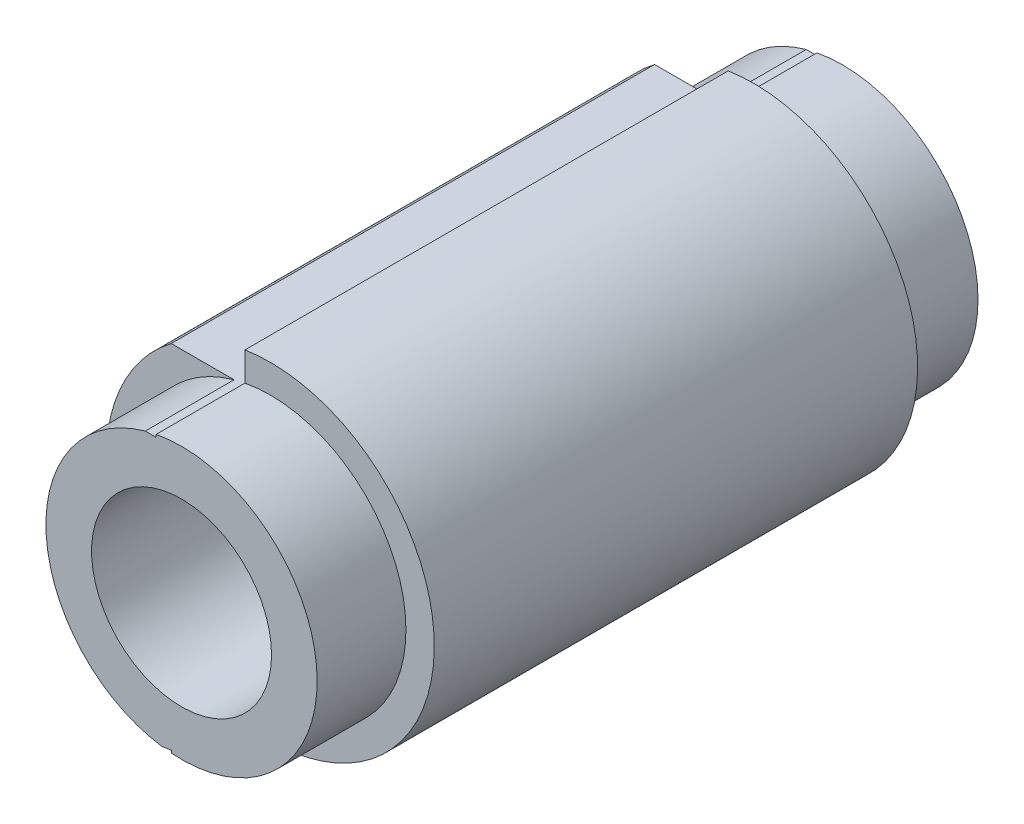
SolidWorks part; units mm, degrees
ref_plane "Front Plane" through (0, 0, 0) normal (0, 0, 1) x (1, 0, 0)
ref_plane "Top Plane" through (0, 0, 0) normal (0, 1, 0) x (1, 0, 0)
ref_plane "Right Plane" through (0, 0, 0) normal (1, 0, 0) x (0, 0, -1)
sketch "Sketch1" plane through (0, 0, 0) normal (0, 0, 1) x (1, 0, 0)
  line L0 (-40.1653, 53) -> (-10.3, 53)
  line L1 (-10.3, 53) -> (-10.3, 65.6975)
  line L2 (0, 0) -> (0, -98.1486) construction
  line L3 (-4.1281, -53.8236) -> (-2.1257, -66.466)
  line L4 (-4.1281, -53.8236) -> (-32.0797, -58.2507)
  circle A0 centre (0, 0) radius 36.5
  arc A1 (-40.1653, 53) -> (-32.0797, -58.2507) centre (0, 0) ccw
  arc A2 (-2.1257, -66.466) -> (-10.3, 65.6975) centre (0, 0) ccw
  dimension "D1" = 73
  dimension "D2" = 133
  dimension "D3" = 53
  dimension "D4" = 10.3
  dimension "D5" = 9
  dimension "D6" = 12.8
  dimension "D7" = 28.3
extrude "Boss-Extrude1" add sketch "Sketch1" along normal blind 268
sketch "Sketch2" plane through (0, 0, 268) normal (0, 0, 1) x (1, 0, 0)
  circle A0 centre (0, 0) radius 55
  circle A1 centre (0, 0) radius 70
  dimension "D1" = 110
  dimension "D2" = 140
extrude "Cut-Extrude1" cut sketch "Sketch2" against normal blind 36
sketch "Sketch3" plane through (0, 0, 0) normal (0, 0, -1) x (-1, 0, 0)
  circle A0 centre (0, 0) radius 55
  circle A1 centre (0, 0) radius 70
  dimension "D1" = 110
  dimension "D2" = 140
extrude "Cut-Extrude2" cut sketch "Sketch3" against normal blind 36
